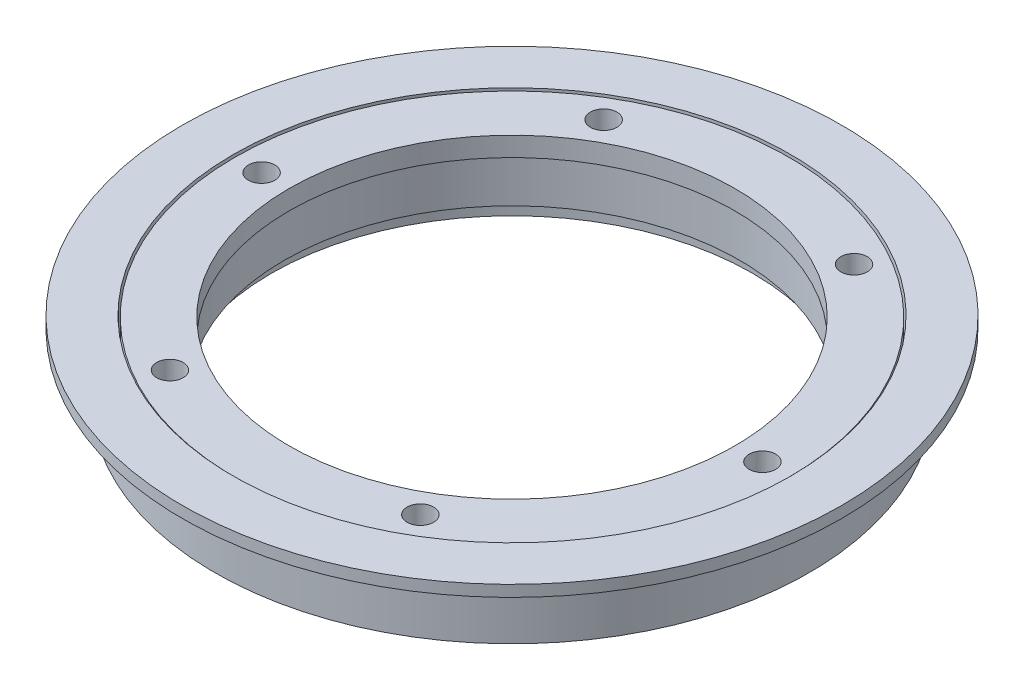
from build123d import *

# Parameters (mm, degrees)
SKETCH2_R          = 2.1
CUT_EXTRUDE1_DEPTH = 68
SKETCH3_R          = 4.1
CUT_EXTRUDE2_DEPTH = 20


with BuildPart() as part:
    # Sketch1 → Revolve1 (revolve)
    with BuildSketch(Plane.XY, mode=Mode.PRIVATE) as revolve1_sk:
        Polygon((92, 154.5), (102, 154.5), (102, 158), (92, 158), (86.24871307, 158), (86.24871307, 135), (92, 135), align=None)
        Polygon((85.742312236, 157.5), (85.742312236, 135), (81.495706961, 135), (81.495706961, 132), (74.495706961, 132), (74.495706961, 137.5), (70.495706961, 137.5), (70.495706961, 151.5), (68.995706961, 151.5), (68.995706961, 157.5), align=None)
    revolve(revolve1_sk.sketch.rotate(Axis((0, 0, 0), (0, -1, 0)), 180), axis=Axis((0, 0, 0), (0, -1, 0)))

    # Sketch2 → Cut-Extrude1 (cut)
    with BuildSketch(Plane.XZ.offset(-132)):
        with Locations((-77.5, 0)):
            Circle(SKETCH2_R)
        with Locations((-38.75, 67.116968793)):
            Circle(SKETCH2_R)
        with Locations((38.75, 67.116968793)):
            Circle(SKETCH2_R)
        with Locations((77.5, 0)):
            Circle(SKETCH2_R)
        with Locations((38.75, -67.116968793)):
            Circle(SKETCH2_R)
        with Locations((-38.75, -67.116968793)):
            Circle(SKETCH2_R)
    extrude(amount=-CUT_EXTRUDE1_DEPTH, mode=Mode.SUBTRACT)

    # Sketch3 → Cut-Extrude2 (cut)
    with BuildSketch(Plane(origin=(0, 157.5, 0), x_dir=(1, 0, 0), z_dir=(0, 1, 0))):
        with Locations(Location((-38.75, -67.116968793, 0), (0, 0, 180))):
            Circle(SKETCH3_R)
        with Locations(Location((-77.5, 0, 0), (0, 0, 180))):
            Circle(SKETCH3_R)
        with Locations(Location((-38.75, 67.116968793, 0), (0, 0, 180))):
            Circle(SKETCH3_R)
        with Locations(Location((38.75, 67.116968793, 0), (0, 0, 180))):
            Circle(SKETCH3_R)
        with Locations(Location((77.5, 0, 0), (0, 0, 180))):
            Circle(SKETCH3_R)
        with Locations(Location((38.75, -67.116968793, 0), (0, 0, 180))):
            Circle(SKETCH3_R)
    extrude(amount=-CUT_EXTRUDE2_DEPTH, mode=Mode.SUBTRACT)


solid = part.part
